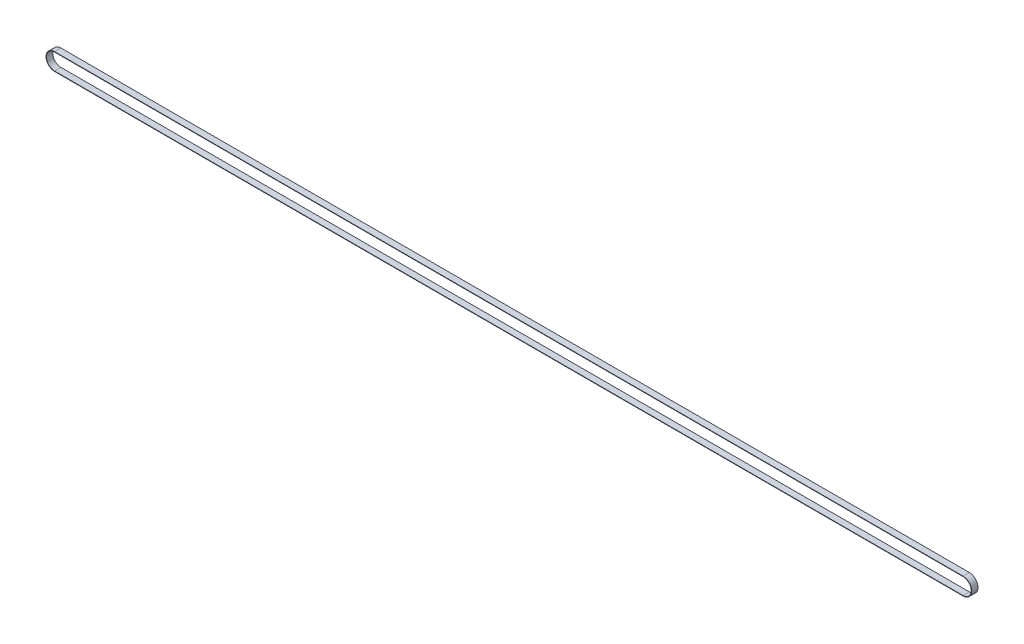
SolidWorks part; units mm, degrees
ref_plane "前视基准面" through (0, 0, 0) normal (0, 0, 1) x (1, 0, 0)
ref_plane "上视基准面" through (0, 0, 0) normal (0, 1, 0) x (1, 0, 0)
ref_plane "右视基准面" through (0, 0, 0) normal (1, 0, 0) x (0, 0, -1)
sketch "草图2" plane through (0, 0, 0) normal (0, 0, 1) x (1, 0, 0)
  line L0 (0, 0) -> (1, 0) construction
  line L1 (0, 0) -> (0, 1) construction
  line L2 (0, 19.415) -> (2155, 19.415)
  line L3 (2155, -19.415) -> (0, -19.415)
  arc A0 (0, -19.415) -> (0, 19.415) centre (0, 0) cw
  arc A1 (2155, 19.415) -> (2155, -19.415) centre (2155, 0) cw
extrude "拉伸-薄壁1" add sketch "草图2" along normal mid plane 15 thin thin type one direction wall 1
